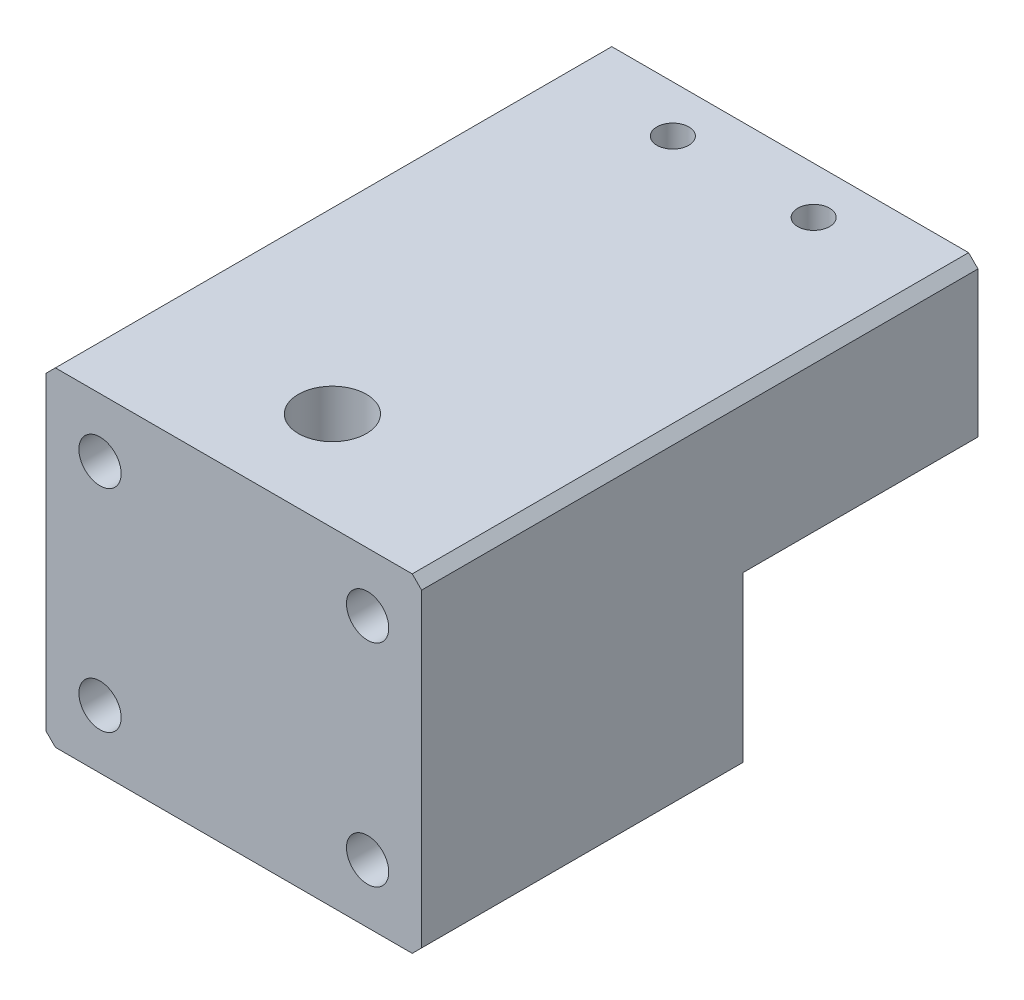
SolidWorks part; units mm, degrees
ref_plane "前视基准面" through (0, 0, 0) normal (0, 0, 1) x (1, 0, 0)
ref_plane "上视基准面" through (0, 0, 0) normal (0, 1, 0) x (1, 0, 0)
ref_plane "右视基准面" through (0, 0, 0) normal (1, 0, 0) x (0, 0, -1)
sketch "草图1" plane through (0, 0, 0) normal (0, 0, 1) x (1, 0, 0)
  line L1 (0, 0) -> (80, 0)
  line L2 (0, 0) -> (0, 70)
  line L3 (0, 70) -> (80, 70)
  line L4 (80, 0) -> (80, 70)
  dimension "D1" = 80
  dimension "D2" = 70
extrude "凸台-拉伸1" add sketch "草图1" along normal blind 118.5
sketch "草图4" plane through (0, 0, 0) normal (0, 0, -1) x (-1, 0, 0)
  circle A0 centre (-11.5, 57.5) radius 7
  circle A1 centre (-11.5, 12.5) radius 7
  circle A2 centre (-68.5, 57.5) radius 7
  circle A3 centre (-68.5, 12.5) radius 7
  dimension "D1" = 14
extrude "切除-拉伸1" cut sketch "草图4" against normal blind 80
sketch "草图5" plane through (0, 0, 0) normal (0, 0, -1) x (-1, 0, 0)
  circle A0 centre (-68.5, 57.5) radius 4.5
  circle A1 centre (-11.5, 57.5) radius 4.5
  circle A2 centre (-11.5, 12.5) radius 4.5
  circle A3 centre (-68.5, 12.5) radius 4.5
  dimension "D1" = 9
extrude "切除-拉伸2" cut sketch "草图5" against normal through all
sketch "草图6" plane through (0, 0, 0) normal (0, 0, -1) x (-1, 0, 0)
  line L0 (0, 70) -> (0, 0) construction
  line L1 (-80, 0) -> (0, 0)
  line L2 (-80, 0) -> (-80, 35)
  line L3 (-80, 35) -> (0, 35)
  line L4 (0, 0) -> (0, 35)
extrude "切除-拉伸3" cut sketch "草图6" against normal blind 50
hole_wizard "M16x1.5 螺纹孔1" positions "草图8" profile "草图9" tap size "M16x1.5" standard "GB"
sketch "草图8" plane through (0, 70, 0) normal (0, 1, 0) x (1, 0, 0)
  line L0 (40, -118.5) -> (40, -44.025) construction
  line L1 (80, -118.5) -> (0, -118.5) construction
  point P0 (40, -97.5)
  dimension "D1" = 21
sketch "草图9" plane through (40, 70, 97.5) normal (1, 0, 0) x (0, 0, 1)
  line L0 (0, 0) -> (0, 40.8562)
  line L1 (0, 40.8562) -> (7.25, 36.5)
  line L2 (7.25, 36.5) -> (7.25, 0)
  line L5 (7.25, 0) -> (0, 0)
  line L10 (0, 40.8562) -> (-7.25, 36.5) construction
  line L11 (0, -6.35) -> (0, 107.95) construction
  dimension "螺纹孔钻头直径" = 14.5
  dimension "螺纹孔钻头深度" = 36.5
  dimension "导头角度" = 118
cosmetic thread "孔螺蚊线1" parameters "D1"=32, "D2"=16
hole_wizard "M8 螺纹孔1" positions "草图11" profile "草图10" tap size "M8" standard "GB"
sketch "草图11" plane through (0, 70, 0) normal (0, 1, 0) x (1, 0, 0)
  point P0 (55, -10)
  point P3 (25, -10)
sketch "草图10" plane through (55, 70, 10) normal (1, 0, 0) x (0, 0, 1)
  line L0 (0, 0) -> (0, 21.7929)
  line L1 (0, 21.7929) -> (3.4, 19.75)
  line L2 (3.4, 19.75) -> (3.4, 0)
  line L5 (3.4, 0) -> (0, 0)
  line L10 (0, 21.7929) -> (-3.4, 19.75) construction
  line L11 (0, -6.35) -> (0, 107.95) construction
  dimension "螺纹孔钻头直径" = 6.8
  dimension "螺纹孔钻头深度" = 19.75
  dimension "导头角度" = 118
cosmetic thread "孔螺蚊线2" parameters "D1"=16, "D2"=8
cosmetic thread "孔螺蚊线3" parameters "D1"=16, "D2"=8
chamfer "倒角1" distance 2 angle 45 6 edges at (0, 70, 59.25) (0, 0, 84.25) (80, 0, 84.25) (80, 70, 59.25) (0, 35, 25) (80, 35, 25)
